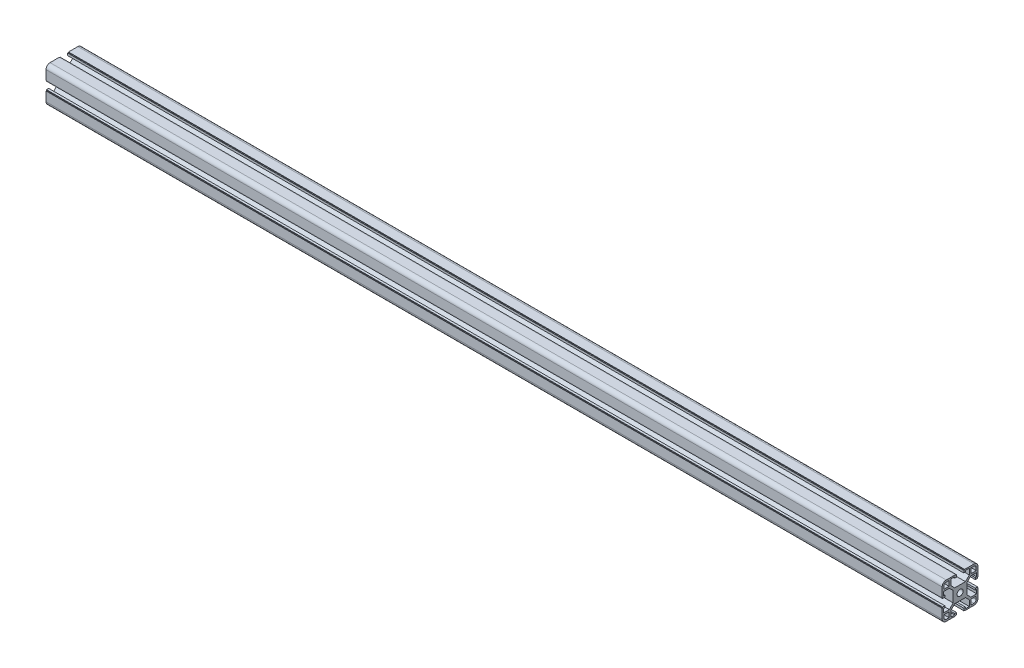
from build123d import *

# Parameters (mm, degrees)
SKETCH1_R                                = 3.4
ALUMINUM_PROFILE_40_X_40B_X_R4_5_1_DEPTH = 1000


with BuildPart() as part:
    # Sketch1 → Aluminum profile 40 X 40B X R4.5(1) (new body)
    with BuildSketch(Plane.YZ):
        with BuildLine():
            Line((-5.1, 20), (-5.1, 19.5))
            Line((-5.1, 19.5), (-4.1, 19.5))
            Line((-4.1, 19.5), (-4.1, 17))
            Line((-4.1, 17), (-6.1, 17))
            Line((-6.1, 17), (-6.1, 18.5))
            Line((-6.1, 18.5), (-10.3, 18.5))
            Line((-10.3, 18.5), (-10.3, 12))
            Line((-10.3, 12), (-6, 7.7))
            Line((-6, 7.7), (6, 7.7))
            Line((6, 7.7), (10.3, 12))
            Line((10.3, 12), (10.3, 18.5))
            Line((10.3, 18.5), (6.1, 18.5))
            Line((6.1, 18.5), (6.1, 17))
            Line((6.1, 17), (4.1, 17))
            Line((4.1, 17), (4.1, 19.5))
            Line((4.1, 19.5), (5.1, 19.5))
            Line((5.1, 19.5), (5.1, 20))
            Line((5.1, 20), (15.5, 20))
            ThreePointArc((15.5, 20), (18.681980515, 18.681980515), (20, 15.5))
            Line((20, 15.5), (20, 5.1))
            Line((20, 5.1), (19.5, 5.1))
            Line((19.5, 5.1), (19.5, 4.1))
            Line((19.5, 4.1), (17, 4.1))
            Line((17, 4.1), (17, 6.1))
            Line((17, 6.1), (18.5, 6.1))
            Line((18.5, 6.1), (18.5, 10.3))
            Line((18.5, 10.3), (12, 10.3))
            Line((12, 10.3), (7.7, 6))
            Line((7.7, 6), (7.7, -6))
            Line((7.7, -6), (12, -10.3))
            Line((12, -10.3), (18.5, -10.3))
            Line((18.5, -10.3), (18.5, -6.1))
            Line((18.5, -6.1), (17, -6.1))
            Line((17, -6.1), (17, -4.1))
            Line((17, -4.1), (19.5, -4.1))
            Line((19.5, -4.1), (19.5, -5.1))
            Line((19.5, -5.1), (20, -5.1))
            Line((20, -5.1), (20, -15.5))
            ThreePointArc((20, -15.5), (18.681980515, -18.681980515), (15.5, -20))
            Line((15.5, -20), (5.1, -20))
            Line((5.1, -20), (5.1, -19.5))
            Line((5.1, -19.5), (4.1, -19.5))
            Line((4.1, -19.5), (4.1, -17))
            Line((4.1, -17), (6.1, -17))
            Line((6.1, -17), (6.1, -18.5))
            Line((6.1, -18.5), (10.3, -18.5))
            Line((10.3, -18.5), (10.3, -12))
            Line((10.3, -12), (6, -7.7))
            Line((6, -7.7), (-6, -7.7))
            Line((-6, -7.7), (-10.3, -12))
            Line((-10.3, -12), (-10.3, -18.5))
            Line((-10.3, -18.5), (-6.1, -18.5))
            Line((-6.1, -18.5), (-6.1, -17))
            Line((-6.1, -17), (-4.1, -17))
            Line((-4.1, -17), (-4.1, -19.5))
            Line((-4.1, -19.5), (-5.1, -19.5))
            Line((-5.1, -19.5), (-5.1, -20))
            Line((-5.1, -20), (-15.5, -20))
            ThreePointArc((-15.5, -20), (-18.681980515, -18.681980515), (-20, -15.5))
            Line((-20, -15.5), (-20, -5.1))
            Line((-20, -5.1), (-19.5, -5.1))
            Line((-19.5, -5.1), (-19.5, -4.1))
            Line((-19.5, -4.1), (-17, -4.1))
            Line((-17, -4.1), (-17, -6.1))
            Line((-17, -6.1), (-18.5, -6.1))
            Line((-18.5, -6.1), (-18.5, -10.3))
            Line((-18.5, -10.3), (-12, -10.3))
            Line((-12, -10.3), (-7.7, -6))
            Line((-7.7, -6), (-7.7, 6))
            Line((-7.7, 6), (-12, 10.3))
            Line((-12, 10.3), (-18.5, 10.3))
            Line((-18.5, 10.3), (-18.5, 6.1))
            Line((-18.5, 6.1), (-17, 6.1))
            Line((-17, 6.1), (-17, 4.1))
            Line((-17, 4.1), (-19.5, 4.1))
            Line((-19.5, 4.1), (-19.5, 5.1))
            Line((-19.5, 5.1), (-20, 5.1))
            Line((-20, 5.1), (-20, 15.5))
            ThreePointArc((-20, 15.5), (-18.681980515, 18.681980515), (-15.5, 20))
            Line((-15.5, 20), (-5.1, 20))
        make_face()
        Circle(SKETCH1_R, mode=Mode.SUBTRACT)
        with BuildLine():
            Line((12.3, 18), (15.5, 18))
            ThreePointArc((15.5, 18), (17.267766953, 17.267766953), (18, 15.5))
            Line((18, 15.5), (18, 12.3))
            Line((18, 12.3), (12.3, 12.3))
            Line((12.3, 12.3), (12.3, 18))
        make_face(mode=Mode.SUBTRACT)
        with BuildLine():
            Line((-15.5, 18), (-12.3, 18))
            Line((-12.3, 18), (-12.3, 12.3))
            Line((-12.3, 12.3), (-18, 12.3))
            Line((-18, 12.3), (-18, 15.5))
            ThreePointArc((-18, 15.5), (-17.267766953, 17.267766953), (-15.5, 18))
        make_face(mode=Mode.SUBTRACT)
        with BuildLine():
            Line((-18, -12.3), (-12.3, -12.3))
            Line((-12.3, -12.3), (-12.3, -18))
            Line((-12.3, -18), (-15.5, -18))
            ThreePointArc((-15.5, -18), (-17.267766953, -17.267766953), (-18, -15.5))
            Line((-18, -15.5), (-18, -12.3))
        make_face(mode=Mode.SUBTRACT)
        with BuildLine():
            Line((12.3, -12.3), (18, -12.3))
            Line((18, -12.3), (18, -15.5))
            ThreePointArc((18, -15.5), (17.267766953, -17.267766953), (15.5, -18))
            Line((15.5, -18), (12.3, -18))
            Line((12.3, -18), (12.3, -12.3))
        make_face(mode=Mode.SUBTRACT)
    extrude(amount=ALUMINUM_PROFILE_40_X_40B_X_R4_5_1_DEPTH)


solid = part.part
